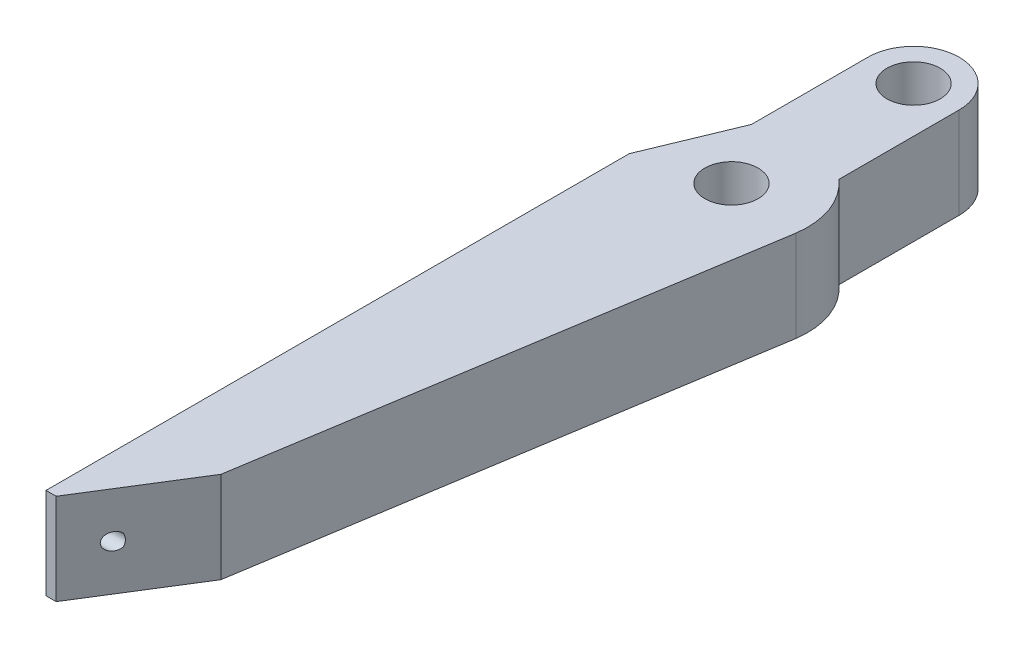
from build123d import *

# Parameters (mm, degrees)
BOSS_EXTRUDE1_DEPTH       = 9
BOSS_EXTRUDE1_DEPTH_BACK  = 9
SKETCH1_R                 = 5.25
M4X0_7_TAPPED_HOLE2_D     = 3.3
M4X0_7_TAPPED_HOLE2_DEPTH = 7.1
M4X0_7_TAPPED_HOLE2_TIP   = 0.991420021


with BuildPart() as part:
    # Sketch1 → Boss-Extrude1 (new, two sides: drawn at the far end of the back side and taken through both)
    with BuildSketch(Plane(origin=(0, 0, 0), x_dir=(1, 0, 0), z_dir=(0, 1, 0)).offset(-BOSS_EXTRUDE1_DEPTH_BACK)):
        with BuildLine():
            Line((0, 0), (0, -115))
            Line((0, -115), (2, -115))
            Line((2, -115), (14.5, -95))
            Line((14.5, -95), (30, 2.863148477))
            ThreePointArc((30, 2.863148477), (29.226286483, 10.190585207), (25.056843998, 16.265592284))
            Line((25.056843998, 16.265592284), (25.056843998, 40))
            ThreePointArc((25.056843998, 40), (16.056843998, 49), (7.056843998, 40))
            Line((7.056843998, 40), (7.056843998, 17.036728487))
            Line((7.056843998, 17.036728487), (0, 0))
        make_face()
        with Locations(Location((16.056843998, 40, 0), (0, 0, 270))):
            Circle(SKETCH1_R, mode=Mode.SUBTRACT)
        with Locations(Location((15.152984624, 5, 0), (0, 0, 270))):
            Circle(SKETCH1_R, mode=Mode.SUBTRACT)
    extrude(amount=BOSS_EXTRUDE1_DEPTH + BOSS_EXTRUDE1_DEPTH_BACK)

    # M4x0.7 Tapped Hole2
    with Locations(Plane(origin=(0, 0, 60), x_dir=(0, 0, -1), z_dir=(-1, 0, 0))):
        with Locations((0, 0), (-48, 0)):
            Hole(M4X0_7_TAPPED_HOLE2_D / 2, depth=M4X0_7_TAPPED_HOLE2_DEPTH)
            with Locations((0, 0, -(M4X0_7_TAPPED_HOLE2_DEPTH + M4X0_7_TAPPED_HOLE2_TIP / 2))):  # 118° drill point
                Cone(0, M4X0_7_TAPPED_HOLE2_D / 2, M4X0_7_TAPPED_HOLE2_TIP, mode=Mode.SUBTRACT)


solid = part.part
